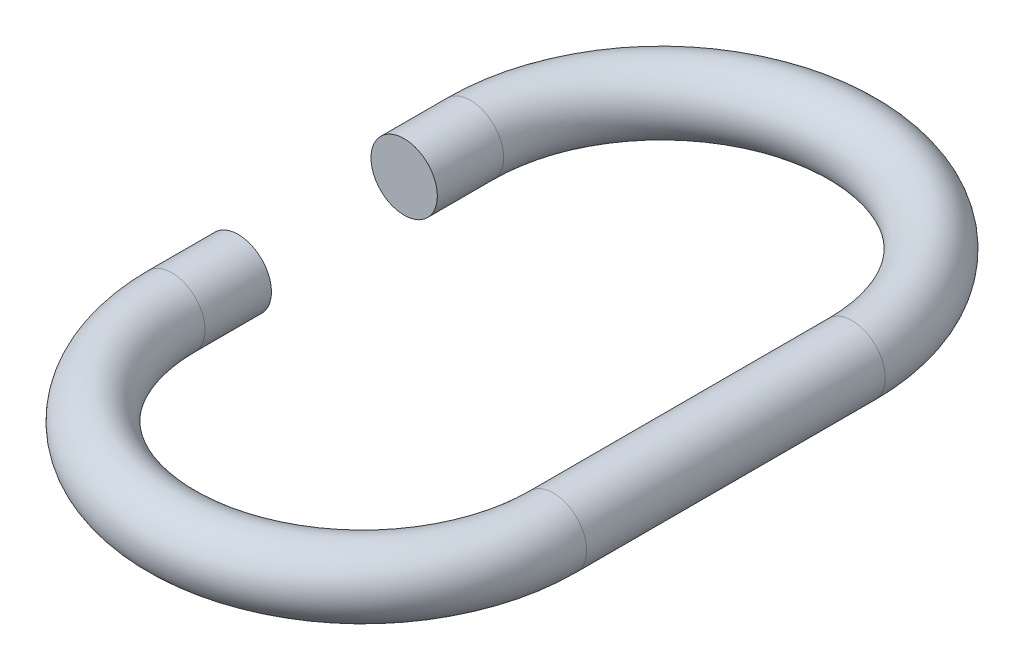
from build123d import *

# Parameters (mm, degrees)
SKETCH2_R = 4


with BuildPart() as part:
    # Sweep1: sweep along a path in Sketch1
    with BuildLine(Plane(origin=(0, 0, 0), x_dir=(1, 0, 0), z_dir=(0, 1, 0))) as sweep1_path:
        Line((-23, 10), (-23, 18))
        ThreePointArc((-23, 18), (0, 41), (23, 18))
        Line((23, 18), (23, -18))
        ThreePointArc((23, -18), (0, -41), (-23, -18))
        Line((-23, -18), (-23, -10))
    # Sketch2 → Sweep1 (sweep)
    with BuildSketch(Plane.XY.offset(-10)):
        with Locations((-23, 0)):
            Circle(SKETCH2_R)
    sweep(path=sweep1_path.line)


solid = part.part
